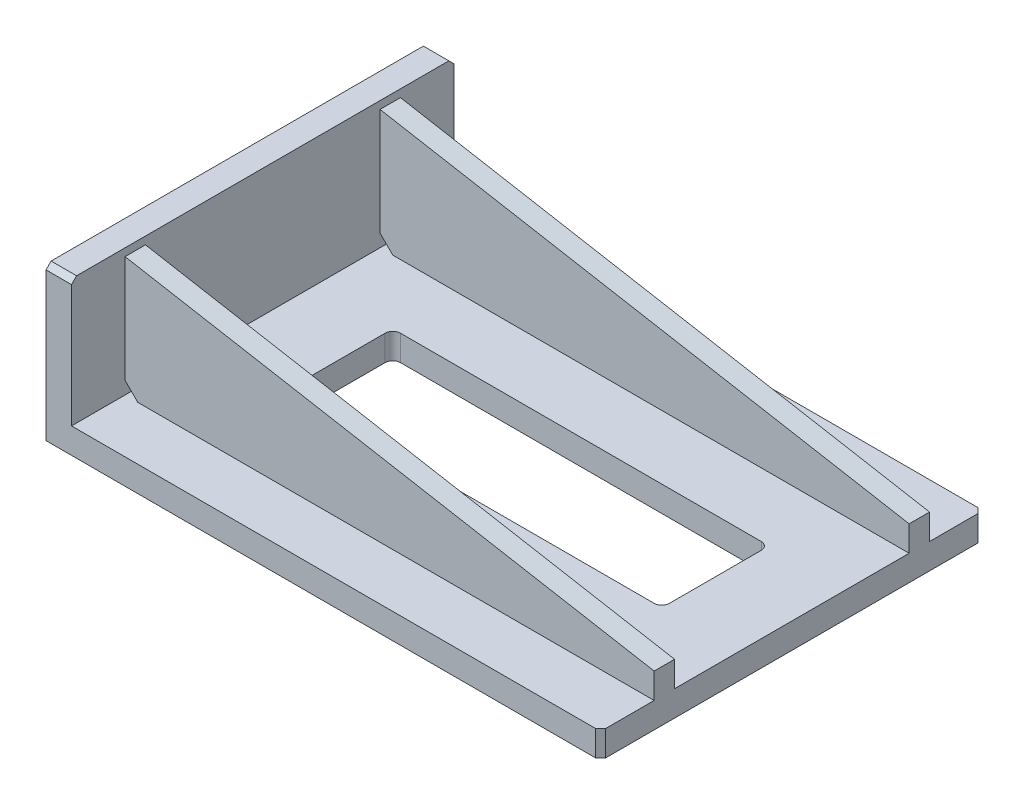
SolidWorks part; units mm, degrees
ref_plane "前视基准面" through (0, 0, 0) normal (0, 0, 1) x (1, 0, 0)
ref_plane "上视基准面" through (0, 0, 0) normal (0, 1, 0) x (1, 0, 0)
ref_plane "右视基准面" through (0, 0, 0) normal (1, 0, 0) x (0, 0, -1)
sketch "草图1" plane through (0, 0, 0) normal (0, 0, 1) x (1, 0, 0)
  line L0 (0, 0) -> (217.5, 0)
  line L1 (217.5, 0) -> (217.5, 10)
  line L2 (217.5, 10) -> (10, 10)
  line L3 (10, 10) -> (10, 60)
  line L4 (10, 60) -> (0, 60)
  line L5 (0, 60) -> (0, 0)
  dimension "D1" = 10
  dimension "D2" = 217.5
  dimension "D3" = 10
  dimension "D4" = 60
extrude "凸台-拉伸1" add sketch "草图1" along normal mid plane 150
sketch "草图2" plane through (0, 0, 0) normal (0, 0, 1) x (1, 0, 0)
  line L0 (10, 57) -> (217.5, 20)
  line L1 (10, 10) -> (10, 60) construction
  line L2 (217.5, 20) -> (217.5, 10)
  line L3 (217.5, 10) -> (10, 10) construction
  line L4 (217.5, 10) -> (15, 10)
  line L5 (15, 10) -> (10, 15)
  line L6 (10, 15) -> (10, 57)
  line L7 (217.5, 0) -> (217.5, 10) construction
  line L8 (10, 60) -> (0, 60) construction
  dimension "D1" = 10
  dimension "D2" = 5
  dimension "D3" = 5
  dimension "D4" = 3
extrude "凸台-拉伸2" add sketch "草图2" along normal mid plane 8 from offset 50
chamfer "倒角1" distance 2 angle 45 4 edges at (217.5, 5, -75) (217.5, 5, 75) (5, 60, 75) (5, 60, -75)
mirror "镜向1" about plane through (0, 0, 0) normal (0, 0, 1) of "凸台-拉伸2"
sketch "草图3" plane through (0, 10, 0) normal (0, 1, 0) x (1, 0, 0)
  line L0 (217.5, 46) -> (10, 46) construction
  line L1 (40, -21) -> (187.5, -21)
  line L2 (40, -21) -> (40, 21)
  line L3 (40, 21) -> (187.5, 21)
  line L4 (187.5, -21) -> (187.5, 21)
  line L5 (40, -21) -> (187.5, 21) construction
  line L6 (40, 21) -> (187.5, -21) construction
  line L7 (10, -75) -> (10, 75) construction
  line L8 (217.5, -46) -> (217.5, 46) construction
  point P0 (113.75, 0)
  point P7 (0, 0)
  dimension "D1" = 25
  dimension "D2" = 30
  dimension "D3" = 30
extrude "切除-拉伸1" cut sketch "草图3" against normal up to next
fillet "圆角1" radius 3 4 edges at (40, 5, 21) (187.5, 5, -21) (187.5, 5, 21) (40, 5, -21)
